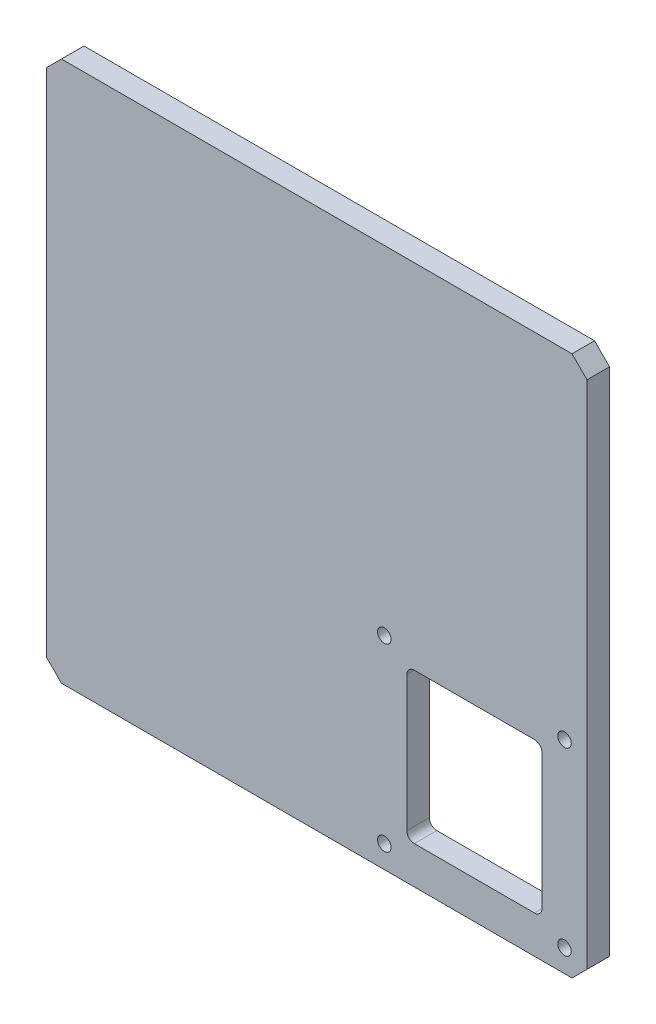
SolidWorks part; units mm, degrees
ref_plane "Front Plane" through (0, 0, 0) normal (0, 0, 1) x (1, 0, 0)
ref_plane "Top Plane" through (0, 0, 0) normal (0, 1, 0) x (1, 0, 0)
ref_plane "Right Plane" through (0, 0, 0) normal (1, 0, 0) x (0, 0, -1)
other "Configuration Table"
sketch "Sketch1" plane through (0, 0, 0) normal (0, 0, 1) x (1, 0, 0)
  line L1 (-180, 180) -> (180, 180)
  line L2 (-180, 180) -> (-180, -180)
  line L3 (-180, -180) -> (180, -180)
  line L4 (180, 180) -> (180, -180)
  line L5 (-180, 180) -> (180, -180) construction
  line L6 (-180, -180) -> (180, 180) construction
  point P0 (0, 0)
  dimension "D1" = 360
  dimension "D2" = 360
extrude "Boss-Extrude1" add sketch "Sketch1" along normal blind 15 contours L1 L4 L3 L2
chamfer "Chamfer1" distance 10 angle 45 4 edges at (-180, -180, 7.5) (180, -180, 7.5) (180, 180, 7.5) (-180, 180, 7.5)
hole_wizard "Ø9.0 (9) Diameter Hole1" positions "Sketch3" profile "Sketch4" hole size "Ø9.0" standard "GB"
sketch "Sketch3" plane through (0, 0, 15) normal (0, 0, 1) x (1, 0, 0)
  line L0 (-170, -180) -> (170, -180) construction
  line L1 (180, 170) -> (180, -170) construction
  point P1 (165, -45)
  point P3 (45, -45)
  point P6 (45, -165)
  point P8 (165, -165)
  dimension "D1" = 120
  dimension "D2" = 120
  dimension "D3" = 15
  dimension "D4" = 15
sketch "Sketch4" plane through (165, -45, 15) normal (1, 0, 0) x (0, -1, 0)
  line L0 (0, 0) -> (0, 22.4539)
  line L1 (0, 22.4539) -> (4.5, 19.75)
  line L2 (4.5, 19.75) -> (4.5, 0)
  line L5 (4.5, 0) -> (0, 0)
  line L10 (0, 22.4539) -> (-4.5, 19.75) construction
  line L11 (0, -6.35) -> (0, 107.95) construction
  dimension "孔直径" = 9
  dimension "孔深度" = 19.75
  dimension "导头角度" = 118
sketch "Sketch5" plane through (0, 0, 15) normal (0, 0, 1) x (1, 0, 0)
  line L0 (45, -45) -> (165, -165) construction
  line L2 (60, -55) -> (150, -55)
  line L3 (60, -55) -> (60, -155)
  line L4 (60, -155) -> (150, -155)
  line L5 (150, -55) -> (150, -155)
  line L6 (60, -55) -> (150, -155) construction
  line L7 (60, -155) -> (150, -55) construction
  point P2 (105, -105)
  dimension "D1" = 100
  dimension "D2" = 90
extrude "Cut-Extrude2" cut sketch "Sketch5" against normal blind 15
fillet "Fillet1" radius 5 4 edges at (150, -155, 7.5) (60, -155, 7.5) (150, -55, 7.5) (60, -55, 7.5)
